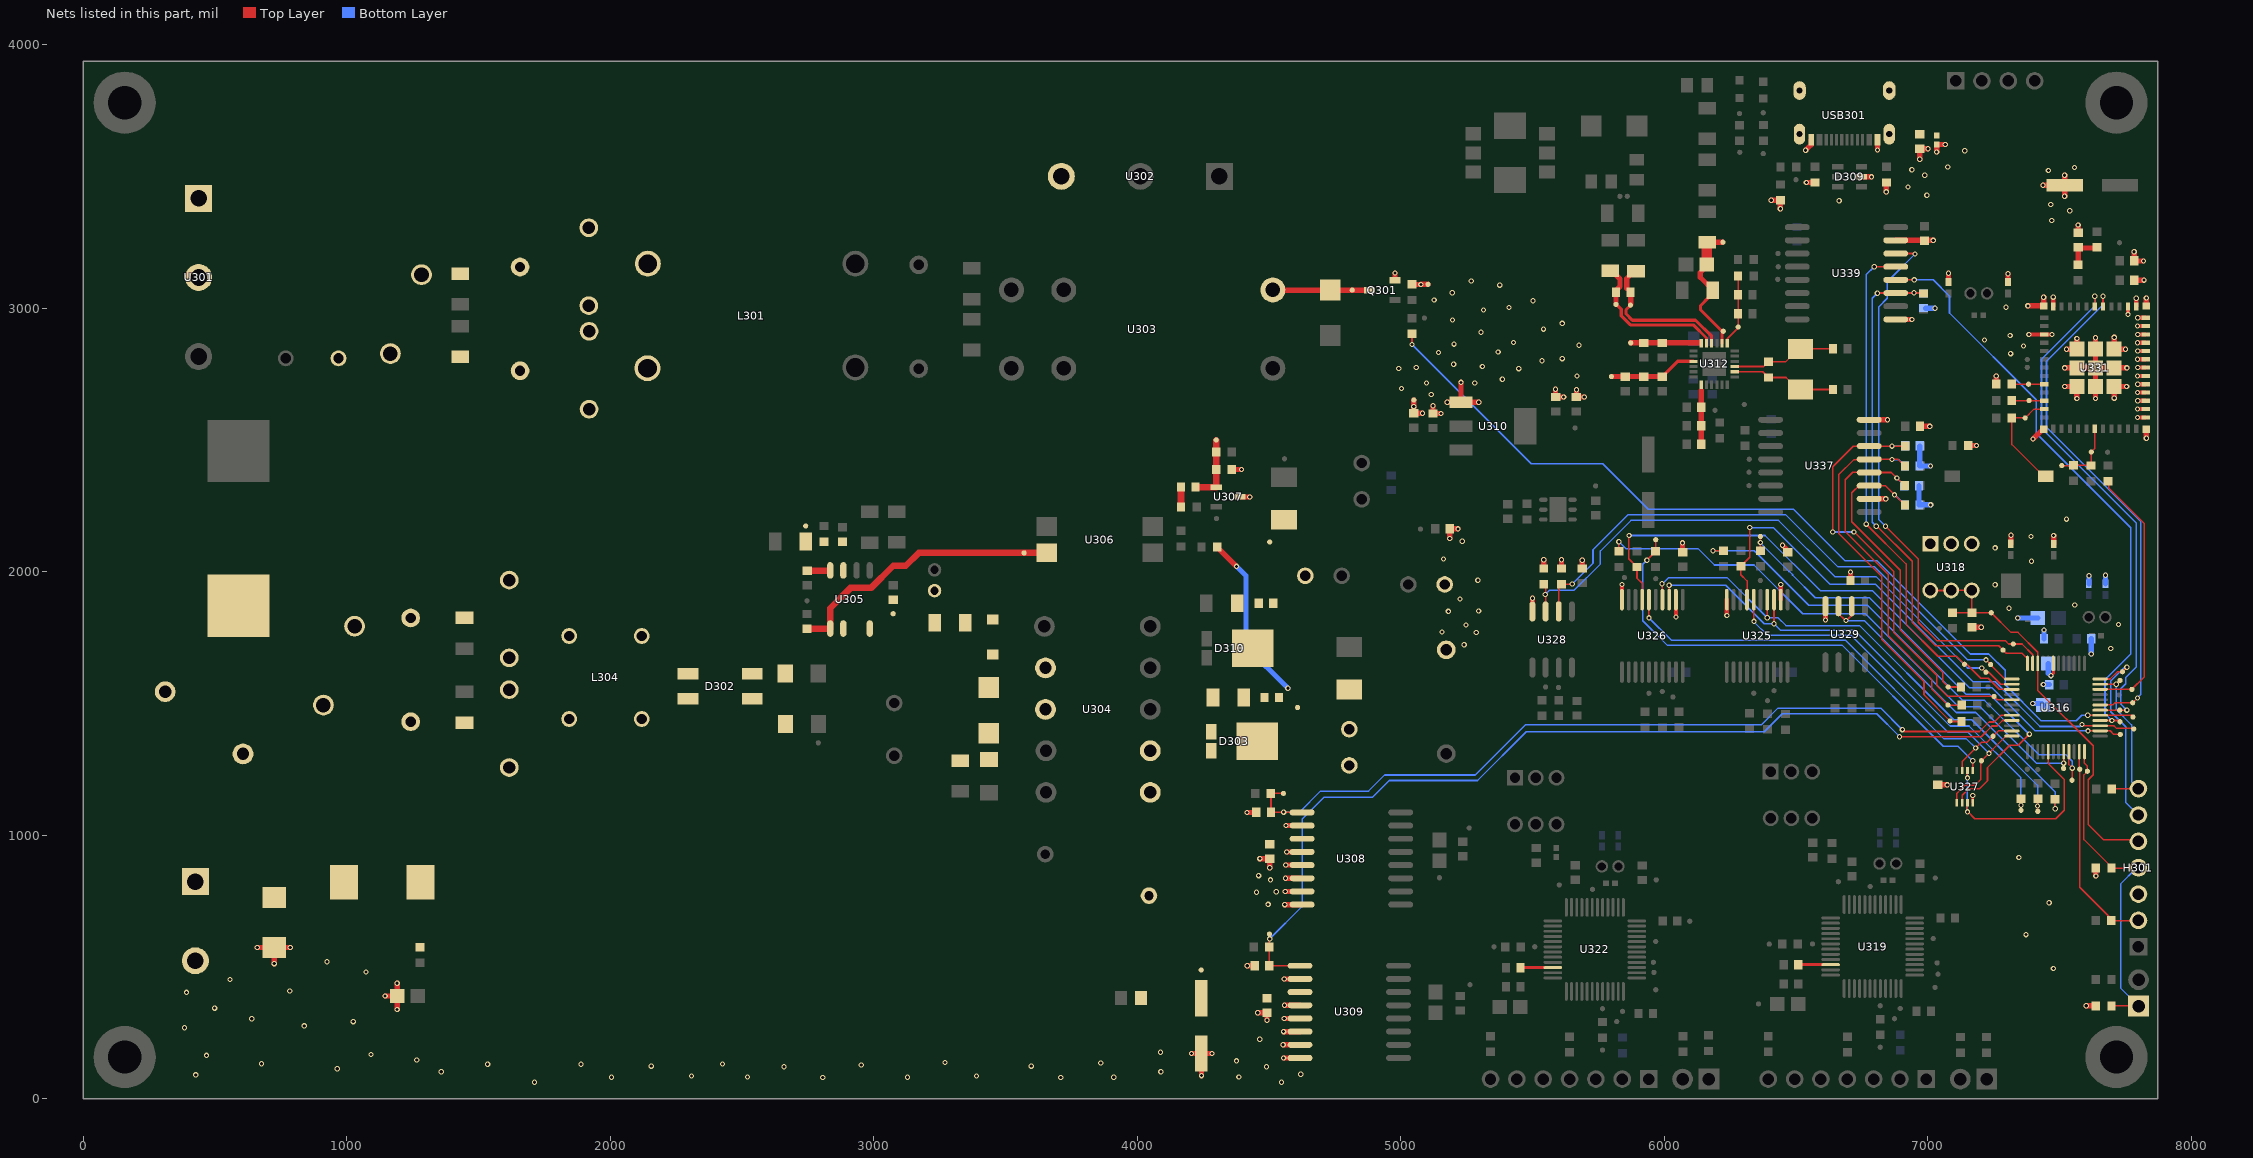
[diagram p0: the nets of this part, all layers, seen from the top]
# Altium PCB MISC84429.PcbDoc (part 3 of 5)
Units mil, origin at the board's own origin, x right, y up, seen from the top; angles counter-clockwise.
Board outline 7874.02 x 3937.01 mil, 4 copper layers (Top Layer, GND, POWER, Bottom Layer); 424 components, 202 nets, 1144 pads, 784 vias.

## Via types
v1: diameter 20, hole 12, Top Layer to Bottom Layer, tented both sides, 695 vias
v2: diameter 20, hole 12, Top Layer to Bottom Layer, 87 vias
v3: diameter 30, hole 15, Top Layer to Bottom Layer, tented both sides, 2 vias

## Nets (pads, with @x,y where several pads share a name; then routed paths per layer and width w, separated by ;. In a path a pad name is that pad's centre, name@x,y a point inside that pad or via, vN(x,y) a via of type N, cw(c..) or ccw(c..) an arc to the next point about the centre after c; other vN are vias at no path point) (continued)
GND: C308.2 C309.2 C311.1 C320.2 C321.1 C322.2 C323.1 C326.1 C327.1 C328.1 C329.1 C332.1 C333.2 C334.1 C335.2 C336.2 C337.2 C338.2 C339.2 C341.2 C358.1 C359.2 C360.2 C361.1 C362.1 C363.2 C364.2 C365.2 C366.1 C367.1 C368.1 C389.2 C391.2 C393.2 C394.2 C396.2 C398.2 C399.1 C400.2 C401.1 C402.1 C403.2 C404.1 C417.2 C419.2 D307.2 D309.2 H301.3 Q301.2 R307.2 R323.1 R356.2 R359.2 R392.2 R394.2 R399.1 R404.2 R406.1 R407.1 R408.1 R409.1 TP303.1 TP304.1 U304.6 U307.3 U308.2 U308.4 U308.5 U308.6 U308.7 U308.8 U309.2 U309.4 U309.5 U309.6 U309.7 U309.8 U310.1 U311.2 U316.7 U318.1 U318.2 U318.3 U325.2 U325.10 U326.2 U326.10 U327.4 U328.4 U329.4 U331.1 U331.2 U331.11 U331.14 U331.36 U331.37 U331.38 U331.39 U331.40 U331.41 U331.42 U331.43 U331.44 U331.45 U331.46 U331.47 U331.48 U331.49 U331.50 U331.51 U331.52 U331.53 U337.2 U337.8 U339.9 U339.15 USB301.1 USB301.12 | length 6349.8
  Top Layer w10: U327.4@7171,1122.97 v1(7171,1150)
  Top Layer w11: v1(7468,1605) 7477.16,1614.16 U316.7@7477.16,1651.32
  Top Layer w16: U326.10@5839.84,1893.44 v1(5839.84,1950.84) ; v1(6044.57,1827.57) U326.2@6044.57,1893.44 ; v1(6237.84,1833.16) U325.10@6237.84,1893.44 ; U325.2@6442.57,1893.44 v1(6442.57,1950.57) ; v1(7384.01,2899.99) U331.14@7442.09,2899.99 v1(7472.01,2899.99) ; U331.11@7476.53,3006.29 v1(7476.53,3041.53) ; v1(7760,2976) U331.2@7760,3006.29 ; U331.1@7791.5,3006.29 v1(7791.5,3037.5) ; v1(7796.48,2585.03) U331.36@7827.91,2585.03 ; v1(7796.48,2616.52) U331.37@7827.91,2616.52 ; v1(7796.48,2679.52) U331.39@7827.91,2679.52 ; v1(7796.48,2742.51) U331.41@7827.91,2742.51 ; v1(7796.48,2805.5) U331.43@7827.91,2805.5 ; v1(7796.48,2868.49) U331.45@7827.91,2868.49 ; v1(7796.48,2931.48) U331.47@7827.91,2931.48 ; v1(7797.02,2648.02) U331.38@7827.91,2648.02 ; v1(7797.02,2711.02) U331.40@7827.91,2711.01 ; v1(7797.02,2774.01) U331.42@7827.91,2774 ; v1(7797.02,2837) U331.44@7827.91,2837 ; v1(7797.02,2899.99) U331.46@7827.91,2899.99 ; v1(7797.02,2962.98) U331.48@7827.91,2962.98
  Top Layer w20: v1(661,573) D307.2@725,573 ; v1(725,512) D307.2@725,573 ; v1(786,573) D307.2@725,573 ; v1(1146,389) C321.1@1191.63,389 ; v1(1191.63,337.63) C321.1@1191.63,389 ; v1(1191.63,437.63) C321.1@1191.63,389 ; v1(4205.89,170.89) C322.2@4243.99,170.89 ; v1(4243.99,86.99) C322.2@4243.99,170.89 ; v1(4284.11,170.89) C322.2@4243.99,170.89 ; R323.1@4359.66,2387 v1(4396,2387) ; U307.3@4389.69,2283 v1(4427,2283) ; v1(4417,1086) C327.1@4452.44,1086 ; v1(4418,504) C326.1@4446.44,504 ; v1(4457.44,325.44) C329.1@4493,325.44 v1(4493,297) ; v1(4465.56,910.44) C323.1@4503,910.44 v1(4503,876) ; v1(4554,204) U309.7@4617.98,204 ; v1(4556,154) U309.8@4617.98,154 ; v1(4556,254) U309.6@4617.98,254 ; v1(4558,304) U309.5@4617.98,304 ; v1(4558,454) U309.2@4617.98,454 ; v1(4559,354) U309.4@4617.98,354 ; v1(4560,736) U308.8@4625.98,736 ; v1(4562,786) U308.7@4625.98,786 ; v1(4563,836) U308.6@4625.98,836 ; v1(4564,886) U308.5@4625.98,886 ; v1(4565,1036) U308.2@4625.98,1036 ; v1(4568,936) U308.4@4625.98,936 ; Q301.2@4978.62,3105.4 v1(4978.62,3132.62) ; R307.2@5043,3089.66 v1(5076.66,3089.66) ; v1(5049.82,2625.82) C333.2@5049.82,2600.75 v1(5082.75,2600.75) ; v1@5050,2627 TP303.1@5050,2651 ; v1@5077,3090 TP304.1@5104,3090 ; v1(5123,2629) C332.1@5123,2599.56 v1(5153.44,2599.56) ; v1(5176.55,2642.55) U310.1@5229,2642.55 ; v1(5186.56,2125.56) C311.1@5186.56,2162 v1(5218,2162) ; v1(5229,2718) U310.1@5229,2642.55 ; v1(5296.55,2642.55) U310.1@5229,2642.55 ; U328.4@5500,1848.5 v1(5500,1899) ; R394.2@5543,2011.66 v1(5543,2045) ; v1(5588,2692) C334.1@5588,2662.56 v1(5618.44,2662.56) ; R392.2@5610,2011.66 v1(5610,2045) ; v1(5667,2690) C335.2@5667,2662.56 v1(5696.56,2662.56) ; C394.2@5689,2011.56 v1(5689,2043) ; C391.2@6070,2073.56 v1(6070,2109) ; v1(6406.34,3409.34) R404.2@6441,3409.34 v1(6441,3377) ; v1(6449,2100) C389.2@6469,2080 ; v1(6537,3599) 6558.01,3620.01 USB301.12@6558.01,3638.49 ; v1(6539.66,3476.34) R408.1@6573,3476.34 ; v1(6612,1816) U329.4@6612,1868.5 ; C396.2@6707.44,1966 v1(6707.44,1998.56) ; D309.2@6749.24,3498 v1(6787,3498) ; U337.2@6778.02,2276 v2(6841,2276) ; U337.8@6778.02,2576 v2(6848,2576) ; v1(6809.99,3599.99) USB301.1@6809.99,3638.49 ; v1(6843,3441) R406.1@6843,3476.34 ; U339.9@6879.02,2957 v2(6940,2957) ; U339.15@6879.02,3257 v2(7021,3257) ; v1(6970,3565) C404.1@6970,3604.88 v1(7000.88,3604.88) ; C417.2@6970.56,2551 v2(7008,2551) ; v1(7034,3592) R409.1@7034,3620.96 v1(7066.96,3620.96) ; C393.2@7038,1190.44 v1(7074.56,1190.44) ; C403.2@7079,3097 C403.2@7079,3098.46 v1(7079,3132) ; R407.1@7153.66,2478 v1(7185,2478) ; C362.1@7168,1788.44 v1(7203.44,1788.44) ; R399.1@7260.34,2711 v1(7260.34,2742.34) ; C402.1@7305,3098.46 v1(7305,3130) ; C360.2@7316,2105.46 v1(7316,2138) ; v1(7380.26,3008.26) U331.52@7440.12,3008.26 v1(7440.12,3041.12) ; v1(7400,2503) 7436.75,2539.75 U331.51@7440.12,2539.75 ; v1(7438.01,3466.01) C398.2@7519.89,3466.01 ; C361.1@7478,2104.46 v1(7478,2137) ; v1(7519.89,3424.11) C398.2@7519.89,3466.01 ; v1(7519.89,3504.11) C398.2@7519.89,3466.01 ; v1(7520.02,2773.02) U331.49@7566.11,2773.02 U331.49@7636.97,2773.02 ; v1(7520.16,2702.16) U331.49@7566.11,2702.16 v1(7566.11,2656.89) ; v1(7527.11,2843.89) U331.49@7566.11,2843.89 v1(7566.11,2884.89) ; C401.1@7571,3285.56 v1(7571,3315) ; v1(7602,352) R356.2@7638.34,352 ; v1(7636.97,2657.03) U331.49@7636.97,2702.16 U331.49@7636.97,2773.02 ; U331.49@7636.97,2830.03 U331.49@7636.97,2773.02 ; U331.49@7636.97,2843.89 v1(7636.97,2887.03) ; v1(7638.34,844.34) R359.2@7638.34,875 ; U331.49@7694.98,2773.02 U331.49@7636.97,2773.02 ; v1(7707.84,2658.16) U331.49@7707.84,2702.16 v1(7755.16,2702.16) ; U331.49@7707.84,2773.02 v1(7755.98,2773.02) ; v1(7707.84,2888.84) U331.49@7707.84,2843.89 v1(7750.89,2843.89) ; C399.1@7783.56,3106 v1(7821,3106) ; v1(7783.56,3213.44) C400.2@7783.56,3179 v1(7819,3179) ; v1(7829.88,2506.12) U331.50@7829.88,2539.75 ; U331.53@7829.88,3008.26 v1(7829.88,3038.12) ; C389.2@6469,2080 C389.2@6469,2073.56 C389.2@6469,2080
  Bottom Layer w20: C337.2@6966.77,2325.86 6966.77,2253.23 v2(7011.23,2253.23) ; C341.2@6968.77,2400.86 v2(7010.86,2400.86) ; C341.2@6969.77,2402.23 C336.2@6969.77,2476.86 ; C339.2@6993,2999 v1(7028,2999) ; v1(7342,1824) C366.1@7417.63,1824 ; v1(7399,1499) 7432.63,1499 C368.1@7438.63,1493 ; v1(7439,1571) C365.2@7461.44,1571 ; C363.2@7441.44,1745 v1(7441.44,1778.44) ; C367.1@7457.63,1651 7457.63,1614.37 v1@7468,1604 ; C358.1@7612,1953.46 v1(7612,1984) ; v1(7620.56,1687.56) C364.2@7620.56,1745 ; C359.2@7675,1953.46 v1(7675,1986)
  other v1: 1713,62 4548,62 2807,80 3710,80 2005,81 3128,81 3911,81 2521,82 4386,82 2309,86 3390,86 427,90 4621,92 1359,102 4090,102 964,113 2660,121 4491,121 2156,123 3598,123 2953,127 1535,130 1889,130 2426,131 677,132 3862,135 3271,137 4376.92,143.08 1266,146 468,164 1092,167 4089,176 4465,225 385,269 839,276 1025,292 640,303 499,343.08 392,403 784,408 557,452 1073,480 925,519 4497,737 4453,783 4528,785 4506,830 4461,846 7695,1708 7724,1799 7309,1861 7558,1873 7256,1950 7394,2039 5163,2048 7256,2090 5234,2115 7392,2133 7527,2199 5116,2672 5003,2695 5098,2716 5281,2716 5386,2730 5669,2742 5448,2770 4993,2771 5059,2774 5310,2778 5201,2787 5536,2800 5613,2808 7315,2827 5144,2831 5370,2833 7364,2856 5677,2859 5202,2863 5428,2869 7216,2879 7313,2896 5305,2908 5542,2920 5613,2942 5197,2955 5314,2993 5411,3002 7297,3003 5502,3028 5127,3031 5196,3058 5376,3087 5268,3103 7471,3332 7539,3369 7467,3393 6664,3407 6997,3428 6925,3459 6989,3504 7458,3522 6940,3525 7557,3533 7076,3535 7141,3597
  other v2: 7477,494 7373,622 7461,743 7346,915 5241,1722 5287,1769 5157,1771 5248,1797 5181,1849 5296,1850 5225,1896 5293,1967
IO8: R396.1 TP423.1 U331.22 | length 122.8
  Top Layer w6: R396.1@7319.66,2649 7320.64,2648.02 U331.22@7442.09,2648.02
IO9: R397.1 SW301.2 TP424.1 U331.23 | length 390.2
  Top Layer w6: SW301.2@7428,2374 7319.66,2482.34 R397.1@7319.66,2583 TP424.1@7370,2583 7403.52,2616.52 U331.23@7442.09,2616.52
IO15_PC0: R399.2 TP422.1 U331.20 | length 122.4
  Top Layer w6: R399.2@7319.66,2711 U331.20@7442.09,2711.01
MCU_CBT6_PA0_ZCR: TP353.1 U316.11 U339.14 | length 2169.9
  Top Layer w6: v2(6840,2172) 6964,2048 6964,1808 7034,1738 7294,1738 7307,1725 TP353.1@7325,1725 7358,1725 7398.42,1684.58 U316.11@7398.42,1651.32 ; 6940,3207 U339.14@6879.02,3207 6950,3207 v2@6952,3209
  Bottom Layer w6: v2(6840,2172) 6814,2198 6814,3004 6847,3037 6847,3100 v2(6952,3205)
MCU_CBT6_PA1_SYN: C339.1 R331.2 TP355.1 U316.12 U339.11 | length 2020.7
  Top Layer w6: v2(6805,2172) 6808,2172 6941,2039 6941,1807 7030,1718 7270,1718 TP355.1@7286,1702 7298,1690 7358,1690 7378.73,1669.27 U316.12@7378.73,1651.32 ; v2@6815,3057 U339.11@6879.02,3057 v2@6948,3057 ; v2(6948,3058) v2@6948,3057 ; R331.2@6970,3057 v2@6948,3057
  Bottom Layer w6: v2(6805,2172) 6790,2187 6790,3037 v2(6809,3056) ; v2(6948,3058) 6976,3058 C339.1@6978,3060
MCU_CBT6_PA4_INT1: TP365.1 U316.15 U339.13 | length 2019.6
  Top Layer w6: v2(6767,2180) 6918,2029 6918,1799 7038,1679 7109,1679 TP365.1@7140,1648 7148,1648 7201,1595 7230,1595 7272.1,1552.9 U316.15@7319.68,1552.9 ; v2@6796,3157 v2(6797,3157) U339.13@6879.02,3157
  Bottom Layer w6: v2(6767,2180) 6767,3127 v2(6797,3157)
MCU_CBT6_PB1_IS3115_EN1: C327.2 R324.1 TP314.1 U308.1 U316.20 | length 3223.6
  Top Layer w6: R324.1@4508,1161 4508,1086 v1@4556,1086 ; R324.1@4518,1158 TP314.1@4555,1158 ; v1(4556,1087) v1@4556,1086 ; U308.1@4625.98,1086 v1@4556,1086 ; v1(6904,1400) 6911,1393 7197,1393 7233,1429 7253,1429 7278.47,1454.47 U316.20@7319.68,1454.47
  Bottom Layer w6: v1@4559,1087 v1(4556,1087) 4616,1087 4696,1167 4878,1167 4939,1228 5283,1228 5473,1418 6368,1418 6432,1482 6822,1482 v1(6904,1400)
MCU_CBT6_PB2_IS3115_EN2: C326.2 R325.1 TP317.1 U309.1 U316.21 | length 3647.9
  Top Layer w6: C326.2@4500,504 4502,506 4502,607 v1(4503,606) ; C326.2@4506,504 U309.1@4617.98,504 ; v1(6893,1373) 7203,1373 7244,1414 7263,1414 7283.79,1434.79 U316.21@7319.68,1434.79
  Bottom Layer w6: v1(4503,606) 4626,729 4626,1060 4709,1143 4893,1143 4957,1207 5268,1207 ; 5276,1207 5268,1207 ; v1@6891,1376 6807,1460 6448,1460 6380,1392 5477,1392 5292,1207 5268,1207
MCU_ESP32-EN: C401.2 R400.1 R401.1 | length 136.6
  Top Layer w20: R401.1@7571,3164.66 7571,3228 7640,3228 R400.1@7643,3231
MCU_ESP32_USART1_CTS: TP348.1 U316.43 U331.5 | length 1956.9
  Top Layer w6: U316.43@7654.32,1493.84 7702.84,1493.84 7711,1502 TP348.1@7778,1502 v1(7796,1520) ; U331.5@7665.51,3006.29 v1(7665.51,3044.51)
  Bottom Layer w6: v1(7665.51,3044.51) 7665.51,3012.51 7451,2798 7451,2548 7808,2191 7808,1532 v1(7796,1520)
MCU_ESP32_USART1_RTS: TP349.1 U316.42 U331.6 | length 1978
  Top Layer w6: U331.6@7634.02,3006.29 v1(7634.02,3045.02) ; U316.42@7654.32,1474.16 TP349.1@7728.84,1474.16 ; TP349.1@7729,1474 v1(7756,1474)
  Bottom Layer w6: v1(7634.02,3045.02) 7634.02,3008.02 7432,2806 7432,2544 7792,2184 7792,1638 7752,1598 7752,1574 7733,1555 7733,1497 v1(7756,1474)
MCU_ESP32_USART1_RX: R403.1 TP344.1 U316.46 | length 987.5
  Top Layer w6: U316.46@7654.32,1552.9 TP344.1@7774.9,1552.9 ; R403.1@7684,2343.34 7684,2343 7687,2340 7687,2317 7822,2182 7822,1600 TP344.1@7775,1553
MCU_ESP32_USART1_TX: R346.1 R398.1 TP347.1 TP426.1 U331.30 | length 256.7
  Top Layer w6: TP347.1@7509,2402 7554.34,2402 7555,2402.66 7621,2402.66 TP426.1@7621,2454 7634.01,2467.01 U331.30@7634.01,2541.72
MCU_G071_IWDG1_IN_PA11: R382.2 TP362.1 U316.33 | length 1871.3
  Top Layer w6: v1(6185,2079) 6226,2079 R382.2@6227,2078 ; U316.33@7536.21,1316.68 7536.21,1267.79 7549,1255 v1(7549,1254) TP362.1@7549,1214
  Bottom Layer w6: v1(6185,2079) 6342,2079 6549,1872 6772,1872 7133,1511 7216,1511 7423,1304 7525,1304 7549,1280 v1(7549,1254)
MCU_G071_IWDG2_IN_PA10: R387.2 TP369.1 U316.32 | length 2130.4
  Top Layer w6: R387.2@5828,2076.66 v1(5828,2113) ; v1(7516,1273) v1@7516.53,1273 ; U316.32@7516.53,1316.68 v1@7516.53,1273 ; TP369.1@7517,1259 7516.53,1259.47 v1@7516.53,1273
  Bottom Layer w6: v1(5828,2113) v1@5828.5,2112.5 ; v1@5829,2113 5856,2086 6130,2086 6191,2025 6341,2025 6526,1840 6764,1840 7117,1487 7199,1487 7413,1273 v1(7516,1273)
MCU_G071_MCO_PA8: R351.1 U329.2 U329.3 | length 1285.4
  Top Layer w6: U329.3@6662,1868.5 6662,1840 v1@6685,1817 ; v1(6690,1814) v1@6693,1814 ; v1@6693,1815 6712,1834 U329.2@6712,1868.5 ; v1(7484,1100) R351.1@7484,1135.34
  Bottom Layer w6: v1@6692,1814 6759,1814 7108,1465 7182,1465 7484,1163 v1(7484,1100)
MCU_G071_PA2_TIM2_CH3_CGT6: R392.1 TP357.1 U316.13 U328.2 | length 2186.9
  Top Layer w6: U328.2@5600,1848.5 R392.1@5600,1942.34 ; R392.1@5610,1952.34 v1@5642.66,1952.34 ; v1(7221,1665) TP357.1@7239,1647 ; TP357.1@7242,1643 7292.73,1592.27 U316.13@7319.68,1592.27
  Bottom Layer w6: v1(5651,1953) 5730,2032 5730,2083 5862,2215 6462,2215 6658,2019 6797,2019 7151,1665 v1(7221,1665)
MCU_G071_PA3_TIM2_CH4_CGT6: R394.1 TP358.1 U316.14 U328.3 | length 2274.6
  Top Layer w6: U328.3@5550,1848.5 R394.1@5550,1945.34 ; v1(7205,1634) TP358.1@7221,1618 7232,1618 7277.42,1572.58 U316.14@7319.68,1572.58
  Bottom Layer w6: v1(5549,1913) 5565,1929 5658,1929 5758,2029 5758,2078 5874,2194 5954,2194 ; 5951,2194 5954,2194 ; v1(7205,1634) 7151,1634 6804,1981 6770.87,1981 6770.43,1980.56 6754.69,1980.56 6754.25,1981 6716.75,1981 6715.31,1979.56 6699.57,1979.56 6698.13,1981 6647,1981 6434,2194 5954,2194
MCU_G071_SPI2_PA9_MISO: U316.29 U327.3 U327.6 | length 829.6
  Top Layer w6: U327.3@7151,1122.97 7151,1090 7179,1062 7486,1062 7518,1094 7518,1211 7457.47,1271.53 U316.29@7457.47,1316.68 ; v1(7151,1217) U327.6@7151,1245.03
  Bottom Layer w6: v1(7151,1088) v1(7151,1217)
MCU_G071_SPI2_PB11_NSS2: TP371.1 U316.23 U326.6 U327.7 | length 1785.2
  Top Layer w6: v1(5942.2,1824.2) U326.6@5942.2,1893.44 ; U327.7@7131,1245.03 7131,1279 v1(7182,1330) 7205,1353 7226,1353 TP371.1@7248,1375 7268.42,1395.42 U316.23@7319.68,1395.42
  Bottom Layer w6: v1@5942,1825 6027,1740 6687,1740 7062,1365 7147,1365 v1(7182,1330)
MCU_G071_SPI2_PB12_NSS1: TP374.1 U316.24 U325.6 U327.1 | length 1554.2
  Top Layer w6: v1@6340.2,1812.2 U325.6@6340.2,1893.44 ; U327.1@7111,1122.97 7111,1159 7141,1189 7179,1189 7201,1211 7201,1279 TP374.1@7204,1282 7297.73,1375.73 U316.24@7319.68,1375.73
  Bottom Layer w6: v1@6341,1809 6392,1758 6709,1758 7077,1390 7153,1390 v1(7233,1310)
  other v1: 6341,1811
MCU_G071_SPI2_PB13_SCK: R353.1 TP376.1 U325.3 U326.3 | length 1928.5
  Top Layer w6: U326.3@6018.98,1893.44 v1(6018.98,1947.98) ; v1(6416.98,1802.02) U325.3@6416.98,1893.44 ; R353.1@7353,1136.34 R353.1@7354,1137.34 v1(7354,1113) TP376.1@7354,1098
  Bottom Layer w6: v1(6018.98,1947.98) 6234.02,1947.98 6379.98,1802.02 v1(6416.98,1802.02) 6441,1778 6721,1778 7085,1414 7157,1414 7354,1217 v1(7354,1113)
MCU_G071_SPI2_PB15_MOSI: R352.1 TP373.1 U325.4 U326.4 | length 2004.1
  Top Layer w6: U326.4@5993.39,1893.44 v1@5993.39,1951.39 ; v1(6391.39,1824.61) U325.4@6391.39,1893.44 ; v1(7417,1110) v1@7418,1110 ; TP373.1@7418,1096 v1@7418,1110 ; R352.1@7418,1137.34 v1@7418,1110
  Bottom Layer w6: v1(5992,1954) 5993,1954 v1@5993.5,1953.5 ; v1@5996,1956 6016,1976 6240,1976 v1(6391.39,1824.61) ; v1@6392,1825 6432,1825 6462,1795 6741,1795 7098.5,1437.5 7167.5,1437.5 7417,1188 v1(7417,1110)
MCU_G071_SPI2_PC6_MISO1: R379.2 TP407.1 U327.2 | length 1773
  Top Layer w6: R379.2@6362,2084 6365,2087 TP407.1@6365,2125 ; U327.2@7131,1122.97 7131,1151 7155,1175 7196,1175 7227,1206 7227,1256 7312,1341 7344,1341 v1(7386,1383)
  Bottom Layer w6: v1@6369,2110 6369,2105 6473.84,2000.16 6476.03,2000.16 6487.16,1989.03 6487.16,1986.84 6573,1901 6779,1901 7145,1535 7234,1535 v1(7386,1383)
  other v1: 6365,2110
MCU_G071_SPI2_PC7_MISO2: R383.2 TP412.1 U327.5 | length 1839.6
  Top Layer w6: v1(5934.34,2043) R383.2@5968,2076.66 TP412.1@5968,2121 ; U327.5@7171,1245.03 v1(7171,1282)
  Bottom Layer w6: 5923,1809 5926,1806 ; v1(5934.34,2043) 5919,2027.66 5919,1813 5926,1806 ; v1@7168,1284 7115,1337 7059,1337 6675,1721 6011,1721 5926,1806 ; v1(7171,1282) v1@7171,1284
MCU_NRST_G071: C362.2 H301.5 R354.1 TP351.1 U316.10 U318.4 U318.5 U318.6 | length 1578.4
  Top Layer w6: U318.4@7009,1928 7095,1928 7095.42,1928.42 U318.6@7167.74,1928.42 ; R354.1@7094,1843.66 7094.1,1843.56 C362.2@7168,1843.56 ; U318.6@7168,1928.16 C362.2@7168,1843.56 ; H301.5@7785,982 7773,982 7667,982 7609,1040 7609,1210 7628,1229 7628,1339 7418.1,1548.9 U316.10@7418.1,1651.32 7418.1,1693.9 7343,1769 7316,1769 TP351.1@7241.44,1843.56 C362.2@7168,1843.56
MCU_PA5_SPI1_SCK: C338.1 R329.2 R348.2 TP361.1 U337.3 | length 1215.8
  Top Layer w6: U337.3@6777,2328 6741,2328 6712,2299 6712,2189 6896,2005 6896,1778 7058,1616 7058,1582 TP361.1@7078,1562 R348.2@7126.34,1562 ; U337.3@6778.02,2326 6840,2326 v2@6874.5,2291.5 ; v2(6874,2291) v2@6874.5,2291.5 ; R329.2@6902,2264 v2@6874.5,2291.5
  Bottom Layer w6: v2@6879,2290 6879,2287.51 C338.1@6913.65,2252.86
MCU_PA6_SPI1_MISO: C336.1 R326.2 TP364.1 U316.17 U337.6 | length 1711
  Top Layer w6: v2@6640,2151 6640,2171 ; 6640,2167 6640,2171 ; v2(6720,2150) 6720,2151 6871,2000 6871,1769 7034,1606 7034,1568 7076,1526 TP364.1@7252,1526 7264.47,1513.53 U316.17@7319.68,1513.53 ; R326.2@6913,2476 v2(6865,2476) U337.6@6778.02,2476 6718,2476 6640,2398 6640,2171
  Bottom Layer w6: v2(6640,2150) v2(6720,2150) ; v2(6865,2476) 6916,2476 C336.1@6917,2477
MCU_PA7_SPI1_MOSI: C337.1 R327.2 R349.2 TP363.1 U337.4 | length 1327.2
  Top Layer w6: U337.4@6756,2377 6716,2377 6687,2348 6687,2152 6851,1988 6851,1756 7015,1592 7015,1555 TP363.1@7077,1493 R349.2@7129.34,1493 ; U337.4@6778.02,2376 6862,2376 v2(6883,2355) R327.2@6908,2330
  Bottom Layer w6: v2(6883,2355) C337.1@6903,2335
MCU_PA13_CBT6_SWDIO: H301.2 R357.1 TP360.1 U316.35 | length 770.9
  Top Layer w6: TP360.1@7575.58,1252.42 U316.35@7575.58,1316.68 ; TP360.1@7577,1250 7577,802 7704,675 H301.2@7783,675
MCU_PA14_CBT6_BOOT0_SWCLK: H301.4 R356.1 R359.1 TP359.1 U316.36 U317.1 | length 1246.3
  Top Layer w6: U316.36@7595,1301 7595,1273 7605,1263 7605,1240 7593,1228 7593,983 7688,888 R359.1@7693,888 ; U316.36@7595.27,1301 U316.36@7595.27,1316.68 ; R359.1@7692,887 7705,874 H301.4@7787,874 ; R356.1@7697.66,352 U317.1@7788,352
  Bottom Layer w6: H301.4@7790,872 7732,814 7732,419.49 U317.1@7800.51,350.98
MCU_PB0_SPI1_CS: C341.1 R332.2 R350.2 TP367.1 U337.5 | length 1448
  Top Layer w6: U337.5@6756,2425 6720,2425 6663,2368 6663,2144 6826,1981 6826,1742 6986,1582 6986,1532 TP367.1@7085,1433 ; U337.5@6778.02,2426 v2@6865,2426 ; v2(6865,2425) v2@6865,2426 ; R332.2@6905,2408 6887,2426 v2@6865,2426 ; TP367.1@7087,1431 R350.2@7128.34,1431
  Bottom Layer w6: v2(6865,2425) 6890,2425 C341.1@6904,2411
MCU_RELAY_CTL_PD3: R306.1 TP350.1 U316.41 | length 3399.8
  Top Layer w6: 5043,2872 R306.1@5043,2902.34 ; v1(7607.53,1454.47) U316.41@7654.32,1454.47 7772.53,1454.47 TP350.1@7779,1448
  Bottom Layer w6: v1@5044,2861 5496,2409 5767,2409 5940,2236 6491,2236 6686,2041 6808,2041 7162,1687 7232,1687 7294,1625 7294,1570 7430,1434 7564,1434 7584.47,1454.47 v1(7607.53,1454.47)
  other v1: 5043,2862
MCU_STPM32_EN_PD2: TP352.1 U316.40 U339.12 | length 2247.1
  Top Layer w6: U339.12@6879.02,3107 v2(6949,3107) ; U316.40@7654.32,1434.79 v1@7699,1434.79 ; v1(7699,1435) v1@7699,1434.79 ; TP352.1@7725.21,1434.79 v1@7699,1434.79
  Bottom Layer w6: v2(6949,3107) 7021,3107 7083,3045 7083,2981 7412,2652 7412,2525 7771,2166 7771,1687 7673,1589 7673,1461 v1(7699,1435)
MCU_U575_NRST_2_EN: R391.2 TP356.1 U316.38 U326.7 | length 2448.5
  Top Layer w6: v1@5866,2138 5866,2048.34 R391.2@5897,2017.34 5897,1975 5916.61,1955.39 U326.7@5916.61,1893.44 ; v1(7608.58,1395.42) U316.38@7654.32,1395.42 7692.58,1395.42 7706,1382 TP356.1@7731,1382
  Bottom Layer w6: v1@5865,2137 v1(5867,2137) 6383,2137 6593,1927 6791,1927 7159,1559 7244,1559 7268.5,1534.5 ; 7265.5,1537.5 7268.5,1534.5 ; v1(7608.58,1395.42) 7407.58,1395.42 7268.5,1534.5
MCU_U575_NRST_EN: R390.2 TP354.1 U316.39 U325.7 | length 2056
  Top Layer w6: U325.7@6314.61,1893.44 6314.61,1964.39 6291,1988 R390.2@6291,2020.34 6325,2054.34 v1(6325,2167) ; v1@7590.9,1415.1 U316.39@7654.32,1415.1 7705.9,1415.1 7715,1406 TP354.1@7779,1406
  Bottom Layer w6: v1@6324,2168 v1(6325,2167) ; v1@6325,2166 6415,2166 6629,1952 6802,1952 7172,1582 7256,1582 7426,1412 7578,1412
  other v1: 7586,1420
MCU_USART3_RX: H301.6 TP342.1 U316.48 | length 755.2
  Top Layer w6: U316.48@7654.32,1592.27 7692.27,1592.27 7720,1620 TP342.1@7739,1620 v1(7756,1637)
  Bottom Layer w6: v1(7756,1637) 7747,1637 7695,1585 7695,1468 7752,1411 7752,1124 H301.6@7799.94,1076.06
MCU_USART3_TX: H301.7 R358.1 TP343.1 U316.47 | length 613.3
  Top Layer w6: U316.47@7654.32,1572.58 v1(7715.58,1572.58) TP343.1@7730,1587 ; R358.1@7698.66,1175 H301.7@7798.88,1175
  Bottom Layer w6: v1(7715.58,1572.58) 7715.58,1476.42 7774,1418 7774,1202 H301.7@7799.94,1176.06
NetC301_1: C301.1 C304.1 L301.1 R302.1 R304.1 R312.1 U301.2
NetC301_2: C301.2 C302.2 F301.2 L301.2 R301.2 R302.2
NetC302_1: C302.1 C304.2 C305.1 C310.2 U301.1 U302.3
NetC305_2: C305.2 C307.2 F302.2 L304.1 R308.2 R310.2
NetC306_1: C306.1 C308.1 D303.3 L302.1 R315.2 TP305.1 | length 647.5
  Top Layer w20: R315.2@4303.66,2093 v2(4377,2019.66)
  Bottom Layer w20: v2@4377,2020 4413,1984 4413,1962 4413,1948 4413,1716 v2(4572,1557)
NetC306_2: C306.2 R309.2
NetC307_1: C307.1 C310.1 L304.4 R310.1 R311.1 R312.2
NetC313_1: C313.1 D305.1 R313.1
NetC314_1: C314.1 C315.1 R314.1 TP309.1 U305.2
NetC316_2: C316.2 TP310.1 U305.1 U306.4 | length 1078.6
  Top Layer w20: U306.4@3643,2071 U306.4@3644,2070
  Top Layer w25: C316.2@2745,1783 2835,1783 U305.1@2835,1783.76 2835,1861 2912,1938 2990,1938 3074,2022 3122,2022 3171,2071 U306.4@3657.21,2071
NetC317_2: C317.2 U305.8 | length 80.6
  Top Layer w25: C317.2@2748,2003.56 U305.8@2828.56,2003.56
NetC318_2: C318.2 R317.2 R321.2 TP308.1 U305.7
NetC319_1: C319.1 R322.2 | length 71.6
  Top Layer w25: R322.2@4166.44,2249.44 C319.1@4166.44,2321
NetC319_2: C319.2 R318.1 R323.2 TP313.1 U307.1 | length 243.1
  Top Layer w25: C319.2@4228.6,2320.6 U307.1@4300.31,2320.6 R318.1@4300.31,2448.31 ; R318.1@4300.34,2454 TP313.1@4300.34,2497.66
NetC322_1: C322.1 C323.2 C329.2 L306.2 TP315.1 U308.3 U309.3
NetC340_1: C340.1 C342.1 C343.2 U312.19 | length 203.2
  Top Layer w20: C340.1@6140.54,2482.54 C342.1@6140.54,2552.79 6140.54,2685.74
NetC344_2: C344.2 R333.2 U312.2 X301.2 | length 400
  Top Layer w6: U312.2@6268.4,2758.47 6373.87,2758.47 R333.2@6396,2736.34 6462.66,2736.34 6508,2691 C344.2@6640.44,2691
NetC348_2: C348.2 R333.1 U312.3 X301.1 | length 400.1
  Top Layer w6: U312.3@6268.4,2778.17 6378.51,2778.17 R333.1@6396,2795.66 6397.34,2797 6462,2797 6511,2846 C348.2@6640.44,2846
NetC349_2: C349.2 C350.2 C351.2 TP331.1 U312.15 | length 335.8
  Top Layer w12: 6093,2797.85 U312.15@6111.58,2797.85
  Top Layer w14: C351.2@5993,2739.56 6051.44,2798 6093,2798
  Top Layer w20: TP331.1@5800,2740 C351.2@5993,2740
NetC352_2: C352.2 C353.2 TP336.1 U312.12 | length 262
  Top Layer w20: TP336.1@5873,2868 U312.12@6135,2868
NetC354_2: C354.2 C355.2 R337.1 TP338.1 U312.7 | length 270.1
  Top Layer w6: U312.7@6239.21,2866.67 6239.21,2883.21 6281,2925 TP338.1@6281,2928 6281,3118 R337.1@6280,3119
NetC356_1: C356.1 R344.1 TP334.1 U312.10 | length 581.5
  Top Layer w12: TP334.1@5870,3008 5855,2993 5855,2978.46 5879.46,2954 6119,2954 6180.16,2892.84 U312.10@6180.16,2866.67 ; TP334.1@5872,3009 TP334.1@5872,3011 TP334.1@5872,3014 ; C356.1@5872,3051 C356.1@5874,3053
  Top Layer w20: TP334.1@5873,3014 5873,3060 5858,3075 5858,3112 5886.55,3140.55 R344.1@5893.1,3140.55
NetC356_2: C356.2 R338.1 TP335.1 U312.11 | length 580.2
  Top Layer w12: TP335.1@5818,3016 5818,3015 5837,2996 5837,2971 5872,2936 6111,2936 6160.47,2886.53 U312.11@6160.47,2866.67
  Top Layer w20: R338.1@5796,3140.78 5801.22,3140.78 5832,3110 5832,3082 5817,3067 TP335.1@5817,3016
NetC357_2: C357.2 R341.1 R343.2 TP333.1 TP340.1 U312.8 | length 497.8
  Top Layer w12: 6138,2992.46 6138,2993 ; R343.2@6168,3043 6168,3039 6138,3009 6138,2993 ; R343.2@6168.5,3042.5 R343.2@6174,3048 ; U312.8@6219.52,2866.67 6219.52,2911.48 6138,2993
  Top Layer w20: R341.1@6161.37,3242.37 6169,3250 TP340.1@6221,3250 ; C357.2@6163.37,3166 6163.37,3160.37 6137,3134 6137,3117 R343.2@6185,3069
  Top Layer w40: C357.2@6161.37,3166 R341.1@6161.37,3242.37
NetC377_1: C377.1 U319.22 | length 118.6
  Top Layer w11: C377.1@6512.9,508.1 U319.22@6631.55,508.1
NetC387_1: C387.1 U322.22 | length 122.9
  Top Layer w11: C387.1@5454.66,497.1 U322.22@5577.55,497.1
NetC404_2: C404.2 R409.2 USB301.13 USB301.14
NetC420_1: C420.1 C423.1 D310.3 L311.1 TP429.1
NetC423_2: C423.2 R432.2
NetD301_2: D301.2 Q301.3 TP301.1 U303.2 | length 348.6
  Top Layer w20: U303.2@4534,3065 4537,3068 TP301.1@4816,3068 Q301.3@4881.38,3068
NetD302_1: D302.1 L303.1
NetD302_2: D302.2 L305.1
NetD302_3: D302.3 L304.2
NetD302_4: D302.4 L304.3
NetD303_1: D303.1 D303.2 R309.1 U304.7
NetD304_1: D304.1 R314.2
NetD304_2: D304.2 U304.2
NetD305_2: D305.2 U304.3 U305.4
NetD306_1: D306.1 F303.2
NetD306_2: D306.2 D307.1 U311.1